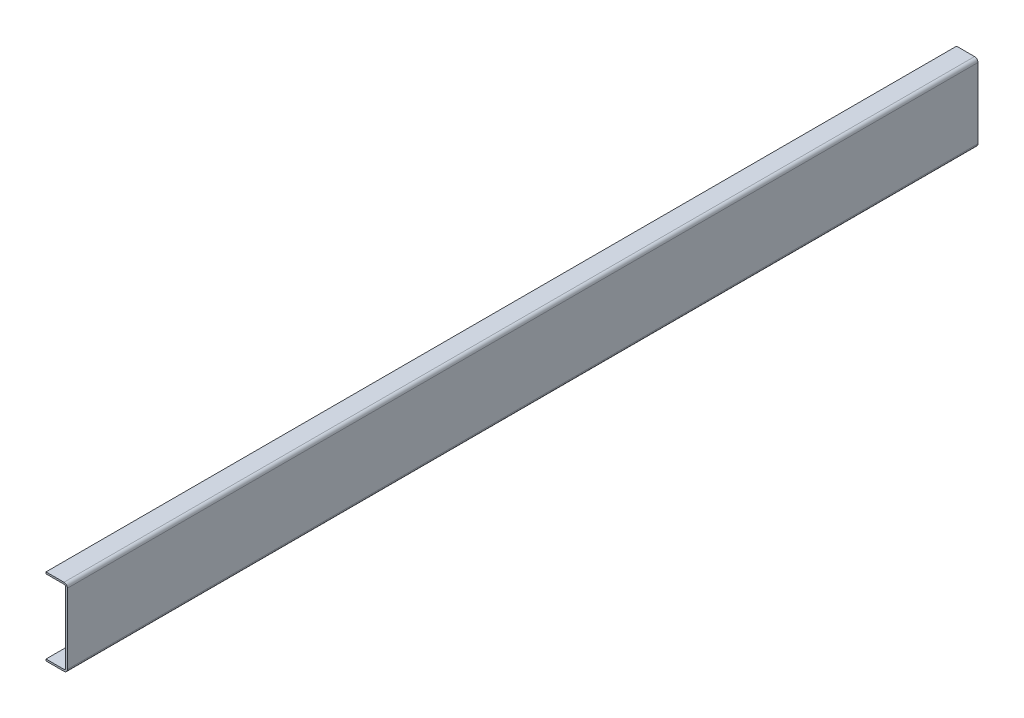
from build123d import *

# Parameters (mm, degrees)
BOSS_EXTRUDE1_DEPTH = 1062


with BuildPart() as part:
    # Sketch1 → Boss-Extrude1 (new, symmetric)
    with BuildSketch(Plane.XY):
        with BuildLine():
            Line((-50, -90), (-8, -90))
            ThreePointArc((-8, -90), (-2.343145751, -87.656854249), (0, -82))
            Line((0, -82), (0, 82))
            ThreePointArc((0, 82), (-2.343145751, 87.656854249), (-8, 90))
            Line((-8, 90), (-50, 90))
            Line((-50, 90), (-50, 86))
            Line((-50, 86), (-8, 86))
            ThreePointArc((-8, 86), (-5.171572875, 84.828427125), (-4, 82))
            Line((-4, 82), (-4, -82))
            ThreePointArc((-4, -82), (-5.171572875, -84.828427125), (-8, -86))
            Line((-8, -86), (-50, -86))
            Line((-50, -86), (-50, -90))
        make_face()
    extrude(amount=BOSS_EXTRUDE1_DEPTH, both=True)


solid = part.part
